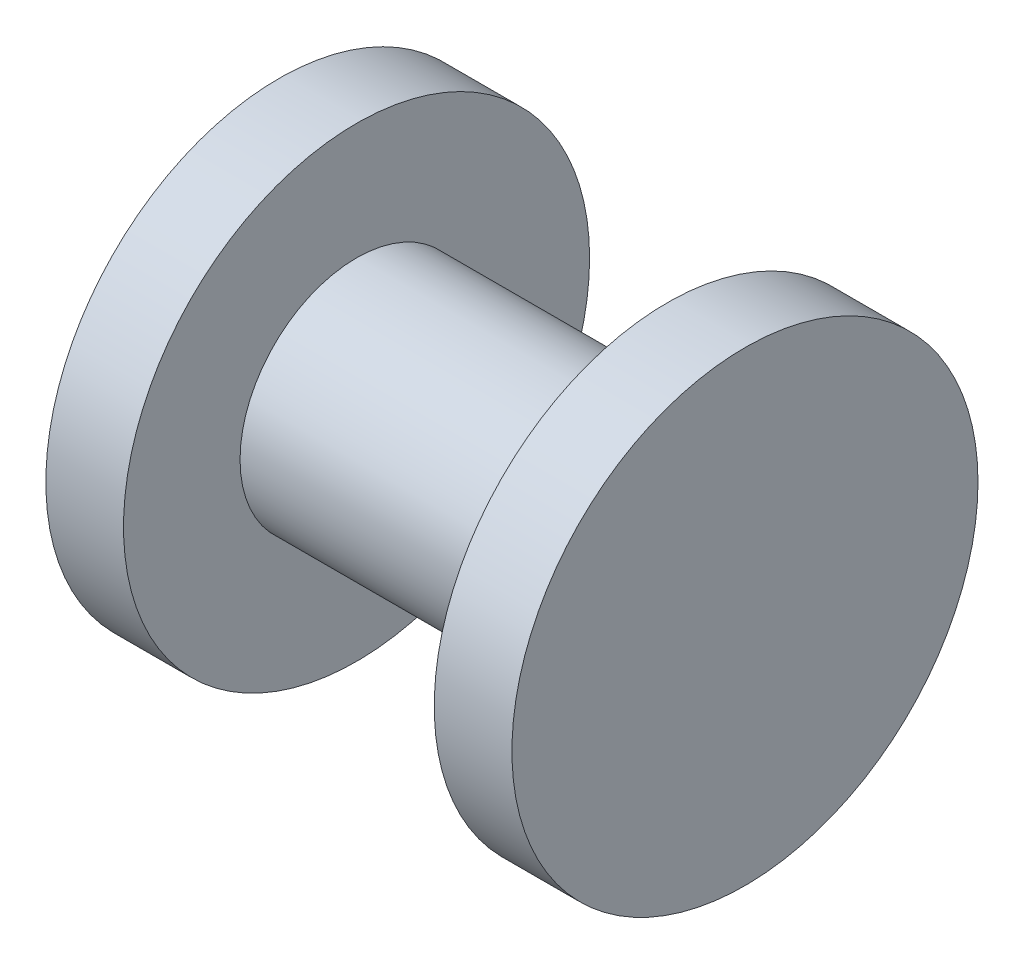
SolidWorks part; units mm, degrees
ref_plane "Front Plane" through (0, 0, 0) normal (0, 0, 1) x (1, 0, 0)
ref_plane "Top Plane" through (0, 0, 0) normal (0, 1, 0) x (1, 0, 0)
ref_plane "Right Plane" through (0, 0, 0) normal (1, 0, 0) x (0, 0, -1)
sketch "Sketch2" plane through (0, 0, 0) normal (0, 0, 1) x (1, 0, 0)
  line L0 (10, -7.5) -> (10, -15)
  line L1 (10, -15) -> (15, -15)
  line L2 (15, -15) -> (15, 0)
  line L3 (15, 0) -> (-15, 0)
  line L4 (-15, 0) -> (-15, -15)
  line L5 (-15, -15) -> (-10, -15)
  line L6 (-10, -15) -> (-10, -7.5)
  line L7 (-10, -7.5) -> (10, -7.5)
revolve "Revolve1" add sketch "Sketch2" angle 360 about L3
scale "Scale1" bodies to scale 107 scale about origin uniform scaling yes scale factor 0.3
